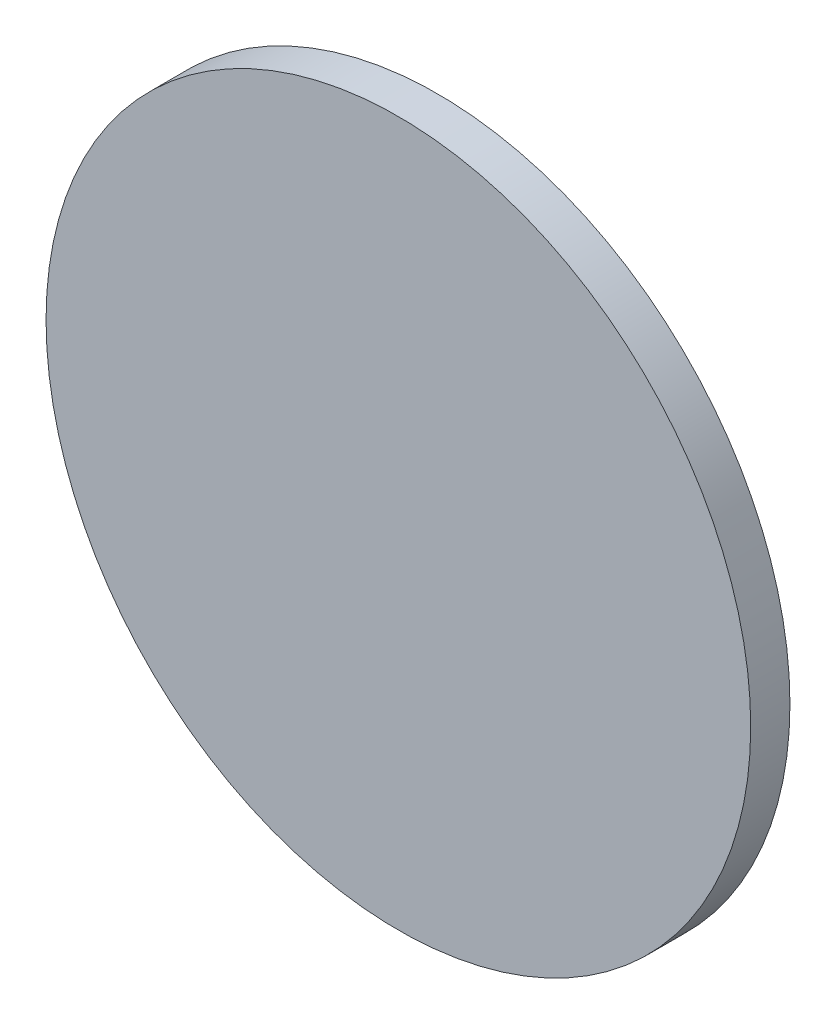
SolidWorks part; units mm, degrees
material "1023 碳钢板 (SS)"
ref_plane "前视基准面" through (0, 0, 0) normal (0, 0, 1) x (1, 0, 0)
ref_plane "上视基准面" through (0, 0, 0) normal (0, 1, 0) x (1, 0, 0)
ref_plane "右视基准面" through (0, 0, 0) normal (1, 0, 0) x (0, 0, -1)
sketch "草图1" plane through (0, 0, 0) normal (0, 0, 1) x (1, 0, 0)
  circle A0 centre (0, 0) radius 26.95
  dimension "D1" = 53.9
extrude "凸台-拉伸1" add sketch "草图1" along normal blind 3 contours A0
